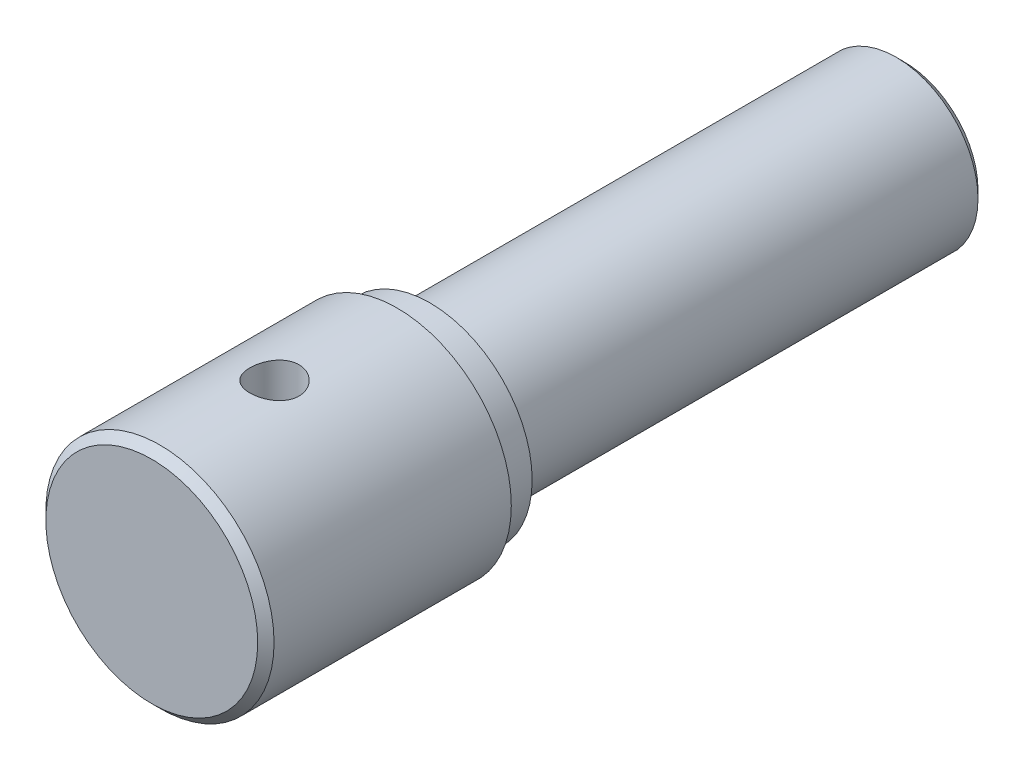
SolidWorks part; units mm, degrees
material "1023 碳钢板 (SS)"
ref_plane "前视基准面" through (0, 0, 0) normal (0, 0, 1) x (1, 0, 0)
ref_plane "上视基准面" through (0, 0, 0) normal (0, 1, 0) x (1, 0, 0)
ref_plane "右视基准面" through (0, 0, 0) normal (1, 0, 0) x (0, 0, -1)
sketch "草图1" plane through (0, 0, 0) normal (0, 0, 1) x (1, 0, 0)
  circle A0 centre (0, 0) radius 10
  dimension "D1" = 20
extrude "凸台-拉伸1" add sketch "草图1" along normal blind 58
sketch "草图2" plane through (0, 0, 58) normal (0, 0, 1) x (1, 0, 0)
  circle A0 centre (0, 0) radius 12.5
  dimension "D1" = 25
extrude "凸台-拉伸2" add sketch "草图2" along normal blind 4
sketch "草图3" plane through (0, 0, 62) normal (0, 0, 1) x (1, 0, 0)
  circle A0 centre (0, 0) radius 13.95
  dimension "D1" = 27.9
extrude "凸台-拉伸3" add sketch "草图3" along normal blind 30
chamfer "倒角1" distance 1 angle 45 2 edges at (10, 0, 0) (13.95, 0, 92)
fillet "圆角1" radius 0.5 1 edges at (10, 0, 58)
sketch "草图4" plane through (0, 0, 0) normal (0, 1, 0) x (1, 0, 0)
  line L0 (13.95, -62) -> (-13.95, -62) construction
  circle A0 centre (0, -77) radius 3
  dimension "D1" = 15
  dimension "D2" = 6
extrude "切除-拉伸1" cut sketch "草图4" against normal mid plane 30
